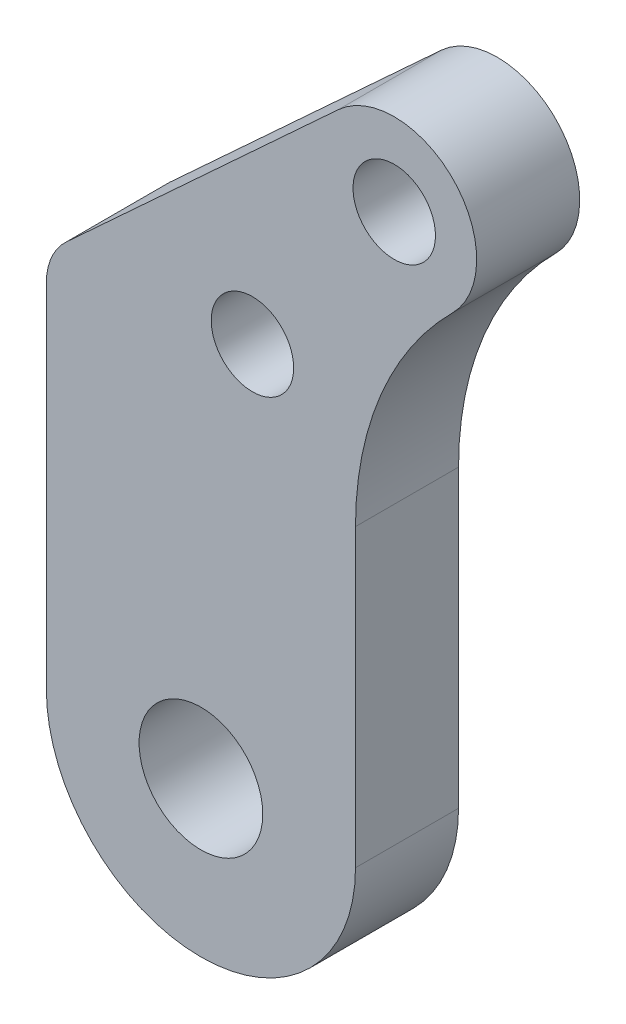
from build123d import *

# Parameters (mm, degrees)
SKETCH1_R           = 3
SKETCH1_R_2         = 2
BOSS_EXTRUDE1_DEPTH = 5


with BuildPart() as part:
    # Sketch1 → Boss-Extrude1 (new body)
    with BuildSketch(Plane.XY):
        with BuildLine():
            Line((-7.5, 0), (-7.5, 17.073921172))
            ThreePointArc((-7.5, 17.073921172), (-7.247513667, 18.278565788), (-6.532554233, 19.280439536))
            Line((-6.532554233, 19.280439536), (6.669927689, 31.442024485))
            ThreePointArc((6.669927689, 31.442024485), (12.26799775, 31.26757457), (12.204, 25.667152669))
            ThreePointArc((12.204, 25.667152669), (8.722720142, 20.47025599), (7.5, 14.335763346))
            Line((7.5, 14.335763346), (7.5, 0))
            ThreePointArc((7.5, 0), (0, -7.5), (-7.5, 0))
        make_face()
        Circle(SKETCH1_R, mode=Mode.SUBTRACT)
        with Locations((2.5, 19.5)):
            Circle(SKETCH1_R_2, mode=Mode.SUBTRACT)
        with Locations((9.38, 28.5)):
            Circle(SKETCH1_R_2, mode=Mode.SUBTRACT)
    extrude(amount=BOSS_EXTRUDE1_DEPTH)


solid = part.part
